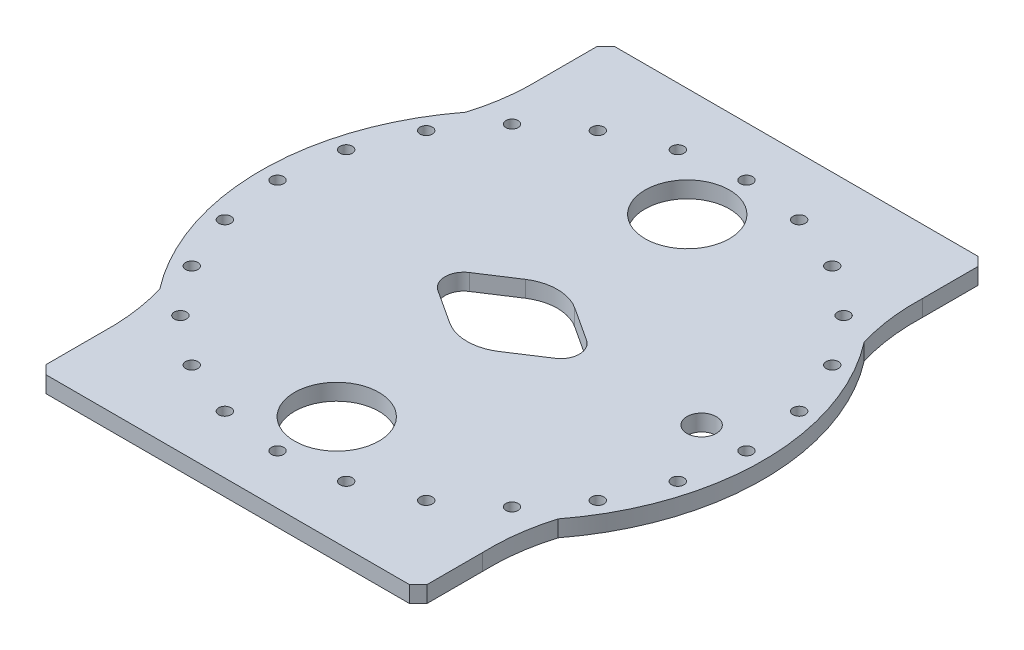
SolidWorks part; units mm, degrees
ref_plane "Front Plane" through (0, 0, 0) normal (0, 0, 1) x (1, 0, 0)
ref_plane "Top Plane" through (0, 0, 0) normal (0, 1, 0) x (1, 0, 0)
ref_plane "Right Plane" through (0, 0, 0) normal (1, 0, 0) x (0, 0, -1)
sketch "Sketch3" plane through (0, 0, 0) normal (0, 1, 0) x (1, 0, 0)
  line L0 (2620.5549, 1673.0679) -> (2562.6769, 1635.306)
  line L1 (2478.6833, 1635.306) -> (2420.8053, 1673.0679)
  line L2 (2420.8053, 1726.7109) -> (2478.6833, 1764.4727)
  line L3 (2562.6769, 1764.4727) -> (2620.5549, 1726.7109)
  line L4 (2845.6801, 2169.5012) -> (2845.6801, 2074.5012)
  line L5 (2845.6801, 2169.5012) -> (2830.6801, 2184.5012)
  line L6 (2210.6801, 2184.5012) -> (2830.6801, 2184.5012)
  line L7 (2195.6801, 2169.5012) -> (2210.6801, 2184.5012)
  line L8 (2195.6801, 2169.5012) -> (2195.6801, 2074.5012)
  line L9 (2195.6801, 1229.5012) -> (2195.6801, 1324.5012)
  line L10 (2210.6801, 1214.5012) -> (2195.6801, 1229.5012)
  line L11 (2210.6801, 1214.5012) -> (2830.6801, 1214.5012)
  line L12 (2845.6801, 1229.5012) -> (2830.6801, 1214.5012)
  line L13 (2845.6801, 1229.5012) -> (2845.6801, 1324.5012)
  circle A0 centre (2844.1801, 1699.5012) radius 25
  circle A1 centre (2520.6801, 1400.5012) radius 72
  circle A2 centre (2520.6801, 1998.5012) radius 72
  arc A3 (2620.5549, 1673.0679) -> (2620.5549, 1726.7109) centre (2603.3611, 1699.8894) ccw
  arc A4 (2478.6833, 1635.306) -> (2562.6769, 1635.306) centre (2520.6801, 1700.2776) ccw
  arc A5 (2420.8053, 1726.7109) -> (2420.8053, 1673.0679) centre (2437.9992, 1699.8894) ccw
  arc A6 (2562.6769, 1764.4727) -> (2478.6833, 1764.4727) centre (2520.6801, 1699.5012) ccw
  arc A7 (2180.8755, 1960.5472) -> (2195.6801, 2074.5012) centre (1842.8877, 2062.3965) ccw
  arc A8 (2180.8755, 1960.5472) -> (2180.8755, 1438.4551) centre (2520.6801, 1699.5012) ccw
  arc A9 (2195.6801, 1324.5012) -> (2180.8755, 1438.4551) centre (1842.8877, 1336.6058) ccw
  arc A10 (2860.4848, 1438.4551) -> (2845.6801, 1324.5012) centre (3198.4725, 1336.6058) ccw
  arc A11 (2860.4848, 1438.4551) -> (2860.4848, 1960.5472) centre (2520.6801, 1699.5012) ccw
  arc A12 (2845.6801, 2074.5012) -> (2860.4848, 1960.5472) centre (3198.4725, 2062.3965) ccw
extrude "Boss-Extrude1" add sketch "Sketch3" along normal blind 28
sketch "Sketch4" plane through (0, 28, 0) normal (0, 1, 0) x (1, 0, 0)
  circle A0 centre (2520.6801, 1699.5012) radius 400 construction
  circle A1 centre (2520.6801, 2099.5012) radius 10.5
  circle A2 centre (2624.2077, 2085.8715) radius 10.5
  circle A3 centre (2720.6801, 2045.9113) radius 10.5
  circle A4 centre (2803.5228, 1982.3439) radius 10.5
  circle A5 centre (2867.0903, 1899.5012) radius 10.5
  circle A6 centre (2907.0504, 1803.0288) radius 10.5
  circle A7 centre (2920.6801, 1699.5012) radius 10.5
  circle A8 centre (2907.0504, 1595.9735) radius 10.5
  circle A9 centre (2867.0903, 1499.5012) radius 10.5
  circle A10 centre (2803.5228, 1416.6585) radius 10.5
  circle A11 centre (2720.6801, 1353.091) radius 10.5
  circle A12 centre (2624.2077, 1313.1308) radius 10.5
  circle A13 centre (2520.6801, 1299.5012) radius 10.5
  circle A14 centre (2417.1525, 1313.1308) radius 10.5
  circle A15 centre (2320.6801, 1353.091) radius 10.5
  circle A16 centre (2237.8374, 1416.6585) radius 10.5
  circle A17 centre (2174.27, 1499.5012) radius 10.5
  circle A18 centre (2134.3098, 1595.9735) radius 10.5
  circle A19 centre (2120.6801, 1699.5012) radius 10.5
  circle A20 centre (2134.3098, 1803.0288) radius 10.5
  circle A21 centre (2174.27, 1899.5012) radius 10.5
  circle A22 centre (2237.8374, 1982.3439) radius 10.5
  circle A23 centre (2320.6801, 2045.9113) radius 10.5
  circle A24 centre (2417.1525, 2085.8715) radius 10.5
  point P53 (2520.6801, 1699.5012)
  dimension "D1" = 800
  dimension "D2" = 21
  dimension "D3" = 24
extrude "Cut-Extrude1" cut sketch "Sketch4" against normal through all
sketch "Sketch6" plane through (0, 0, 0) normal (0, -1, 0) x (1, 0, 0)
  line L0 (2758.1801, -2129.5012) -> (2283.1801, -2129.5012)
  line L1 (2758.1801, -1259.5012) -> (2283.1801, -1259.5012)
  line L2 (2758.1801, -1259.5012) -> (2758.1801, -2139.5012)
  line L3 (2758.1801, -2139.5012) -> (2283.1801, -2139.5012)
  line L4 (2283.1801, -1259.5012) -> (2283.1801, -2139.5012)
  line L5 (2758.1801, -1259.5012) -> (2283.1801, -2139.5012) construction
  line L6 (2758.1801, -2139.5012) -> (2283.1801, -1259.5012) construction
  line L7 (2758.1801, -1269.5012) -> (2283.1801, -1269.5012)
  point P0 (2520.6801, -1699.5012)
  dimension "D1" = 880
  dimension "D2" = 475
  dimension "D3" = 10
  dimension "D4" = 10
